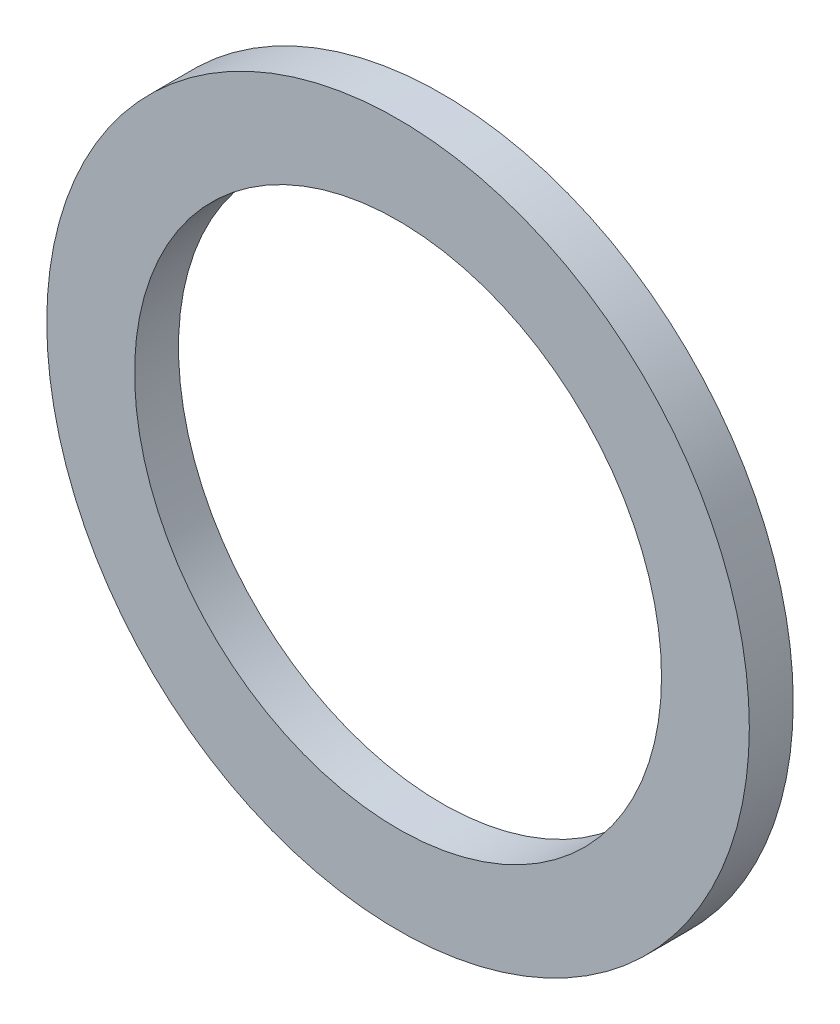
SolidWorks part; units mm, degrees
material "1023 碳钢板 (SS)"
ref_plane "前视基准面" through (0, 0, 0) normal (0, 0, 1) x (1, 0, 0)
ref_plane "上视基准面" through (0, 0, 0) normal (0, 1, 0) x (1, 0, 0)
ref_plane "右视基准面" through (0, 0, 0) normal (1, 0, 0) x (0, 0, -1)
sketch "草图1" plane through (0, 0, 0) normal (0, 0, 1) x (1, 0, 0)
  circle A0 centre (0, 0) radius 3
  circle A1 centre (0, 0) radius 4
  dimension "D1" = 6
  dimension "D2" = 8
extrude "凸台-拉伸1" add sketch "草图1" along normal blind 0.5
